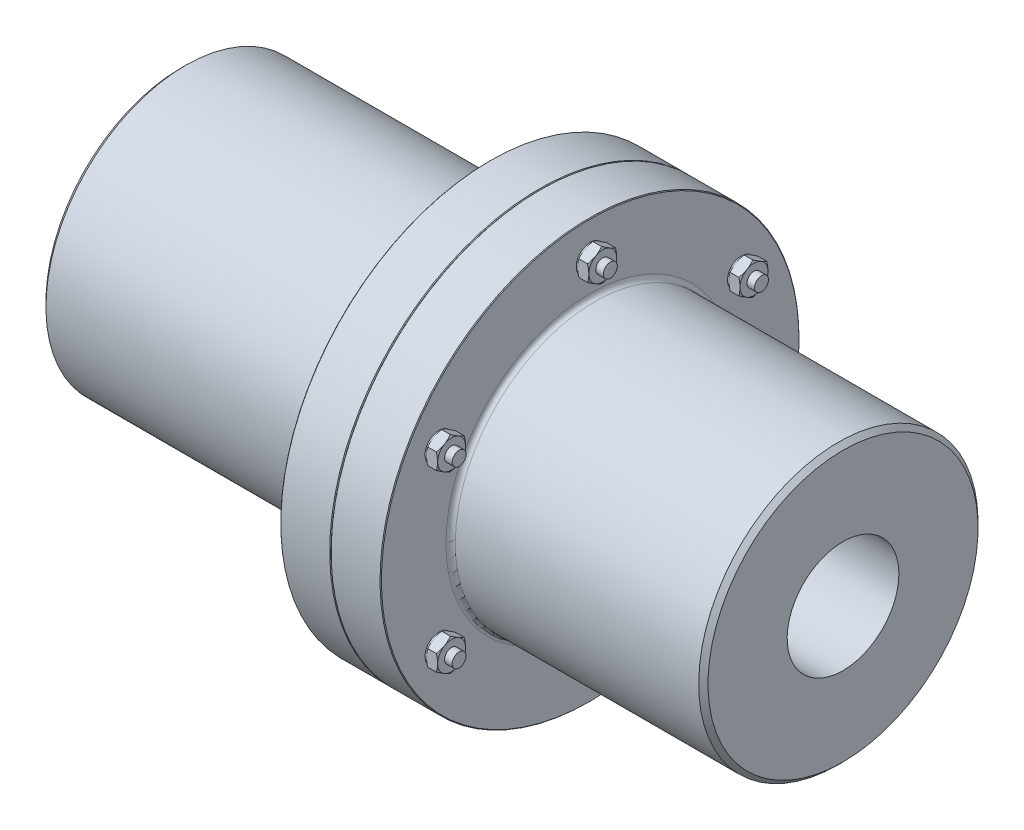
SolidWorks part; units mm, degrees
ref_plane "Front Plane" through (0, 0, 0) normal (0, 0, 1) x (1, 0, 0)
ref_plane "Top Plane" through (0, 0, 0) normal (0, 1, 0) x (1, 0, 0)
ref_plane "Right Plane" through (0, 0, 0) normal (1, 0, 0) x (0, 0, -1)
sketch "Sketch1" plane through (0, 0, 0) normal (0, 0, 1) x (1, 0, 0)
  line L0 (-257, 0) -> (217, 0) construction
  line L1 (0, 0) -> (0, 150) construction
  line L2 (36, 150) -> (-36, 150)
  line L3 (-36, 150) -> (-36, 100)
  line L4 (-36, 100) -> (-257, 100)
  line L5 (-257, 100) -> (-257, 0)
  line L6 (5, 105) -> (-5, 105)
  line L7 (-5, 105) -> (-5, 0)
  line L8 (-5, 65) -> (-257, 65)
  line L9 (-257, 66) -> (-256, 65)
  line L10 (-256, 65) -> (-256, 0)
  line L11 (-257, 2) -> (-5, 2)
  line L12 (36, 150) -> (36, 100)
  line L13 (217, 2) -> (5, 2)
  line L14 (216, 60) -> (216, 0)
  line L15 (217, 61) -> (216, 60)
  line L16 (5, 60) -> (217, 60)
  line L17 (5, 105) -> (5, 0)
  line L18 (217, 100) -> (217, 0)
  line L19 (36, 100) -> (217, 100)
  line L20 (-36, 125) -> (36, 125) construction
  line L21 (-36, 130) -> (36, 130)
  point P29 (0, 105)
  dimension "L" = 252
  dimension "S" = 10
  dimension "d1" = 130
  dimension "(D1)" = 200
  dimension "b" = 72
  dimension "D" = 300
  dimension "D22" = 250
  dimension "沉孔d1" = 210
  dimension "D4" = 1
  dimension "D5" = 45
  dimension "D6" = 4
  dimension "D7" = 1
  dimension "螺母d" = 10
  dimension "d2" = 120
  dimension "D8" = 45
  dimension "L2" = 212
sketch "Sketch14" plane through (0, 0, 0) normal (1, 0, 0) x (0, 0, -1)
  line L0 (0, 0) -> (-72.4, 0) construction
  line L1 (-72.4, 0) -> (-72.4, 16)
  line L2 (-72.4, 16) -> (-63, 16)
  line L3 (0, 0) -> (0, 150) construction
  line L4 (0, 0) -> (0, 150) construction
  line L6 (72.4, 16) -> (63, 16)
  line L7 (72.4, 0) -> (72.4, 16)
  line L8 (0, 0) -> (-36.2, -62.7002) construction
  line L9 (0, 0) -> (65, 0) construction
  line L10 (-36.2, -62.7002) -> (-50.0564, -54.7002)
  line L11 (-50.0564, -54.7002) -> (-45.3564, -46.5596)
  line L12 (0, 0) -> (32.5, 56.2917) construction
  circle A0 centre (0, 0) radius 65
  point P4 (-65, 0)
  point P12 (65, 0)
  dimension "D1" = 120
  dimension "b1" = 32
  dimension "t1" = 137.4
  dimension "B型t" = 137.4
  dimension "B型b" = 32
sketch "Sketch2" plane through (0, 0, 0) normal (0, 0, 1) x (1, 0, 0)
  line L0 (-257, 100) -> (-257, 0) construction
  line L1 (-36, 100) -> (-257, 100) construction
  line L2 (-36, 150) -> (-36, 100) construction
  line L3 (36, 150) -> (-36, 150) construction
  line L4 (0, 0) -> (0, 150) construction
  line L5 (5, 105) -> (-5, 105) construction
  line L6 (-5, 105) -> (-5, 0) construction
  line L8 (-257, 100) -> (-257, 0)
  line L9 (-36, 100) -> (-257, 100)
  line L10 (-36, 150) -> (-36, 100)
  line L11 (0, 150) -> (-36, 150)
  line L12 (0, 105) -> (0, 150)
  line L13 (0, 105) -> (-5, 105)
  line L14 (-5, 105) -> (-5, 0)
  line L15 (-257, 0) -> (-5, 0)
  line L18 (-257, 0) -> (217, 0) construction
  line L21 (-257, 0) -> (217, 0) construction
revolve "Revolve1" add sketch "Sketch2" angle 360 mid plane about L21
chamfer "Chamfer1" distance 3.3333 angle 45 1 edges at (-257, -100, 0)
chamfer "Chamfer2" distance 0.5 angle 45 2 edges at (0, -150, 0) (-36, -150, 0)
fillet "Fillet1" radius 1 1 edges at (-36, -100, 0)
sketch "Sketch15" plane through (0, 0, 0) normal (1, 0, 0) x (0, 0, -1)
  circle A0 centre (0, 0) radius 65 construction
  circle A1 centre (0, 0) radius 65
extrude "Cut-Extrude5" cut sketch "Sketch15" against normal through all
sketch "Sketch20" plane through (0, 0, 0) normal (1, 0, 0) x (0, 0, -1)
  line L0 (72.4, 16) -> (63, 16) construction
  line L1 (72.4, 0) -> (72.4, 16) construction
  line L2 (0, 0) -> (65, 0) construction
  line L3 (72.4, 16) -> (63, 16)
  line L4 (72.4, -16) -> (72.4, 16)
  line L5 (0, 0) -> (65, 0) construction
  line L6 (72.4, -16) -> (63, -16)
  circle A0 centre (0, 0) radius 65 construction
  circle A1 centre (0, 0) radius 65
extrude "Cut-Extrude7" cut sketch "Sketch20" against normal through all contours A1 L6 L4 L3
sketch "Sketch22" [suppressed] plane through (0, 0, 0) normal (1, 0, 0) x (0, 0, -1)
  line L0 (0, 0) -> (-6.15, -10.6521) construction
  line L1 (-8.7481, -9.1521) -> (-7.105, -6.3062) construction
  line L2 (-6.15, -10.6521) -> (-8.7481, -9.1521) construction
  line L3 (0, 0) -> (-6.15, -10.6521) construction
  line L4 (-8.7481, -9.1521) -> (-7.105, -6.3062)
  line L5 (-3.5519, -12.1521) -> (-8.7481, -9.1521)
  line L6 (-3.5519, -12.1521) -> (-1.9089, -9.3062)
  circle A0 centre (0, 0) radius 9.5 construction
  circle A1 centre (0, 0) radius 9.5
extrude "Cut-Extrude8" [suppressed] cut sketch "Sketch22" against normal through all contours L3 A1 L4 L5 | A1 L3 L5 L6
sketch "Sketch23" [suppressed] plane through (0, 0, 0) normal (1, 0, 0) x (0, 0, -1)
  line L0 (-12.3, 3) -> (-9.0139, 3) construction
  line L1 (-12.3, 0) -> (-12.3, 3) construction
  line L2 (0, 0) -> (-12.3, 0) construction
  line L3 (-12.3, 3) -> (-9.0139, 3)
  line L4 (-12.3, -3) -> (-12.3, 3)
  line L5 (0, 0) -> (-12.3, 0) construction
  line L6 (-12.3, -3) -> (-9.0139, -3)
  circle A0 centre (0, 0) radius 9.5 construction
  circle A1 centre (0, 0) radius 9.5
extrude "Cut-Extrude9" [suppressed] cut sketch "Sketch23" against normal through all contours L5 A1 L3 L4 | A1 L5 L4 L6
sketch "Sketch3" plane through (0, 0, 0) normal (0, 0, 1) x (1, 0, 0)
  line L0 (36, 150) -> (-36, 150) construction
  line L1 (36, 150) -> (36, 100) construction
  line L2 (36, 100) -> (217, 100) construction
  line L3 (217, 100) -> (217, 0) construction
  line L4 (5, 105) -> (-5, 105) construction
  line L5 (5, 105) -> (5, 0) construction
  line L9 (36, 150) -> (0, 150)
  line L10 (36, 150) -> (36, 100)
  line L11 (36, 100) -> (217, 100)
  line L12 (217, 100) -> (217, 60)
  line L13 (5, 105) -> (0, 105)
  line L14 (5, 105) -> (5, 0)
  line L15 (5, 0) -> (217, 0)
  line L16 (-257, 0) -> (217, 0) construction
  line L17 (217, 60) -> (217, 0)
  line L18 (0, 150) -> (0, 105)
  line L19 (-257, 0) -> (217, 0) construction
revolve "Revolve2" add sketch "Sketch3" angle 360 mid plane about L19
sketch "Sketch16" plane through (0, 0, 0) normal (1, 0, 0) x (0, 0, -1)
  line L0 (0, 0) -> (-33.7, -58.3701) construction
  line L1 (0, 0) -> (-150, 0) construction
  line L2 (-67.4, -16) -> (-67.4, 16) construction
  line L3 (-67.4, 16) -> (-57.8273, 16) construction
  line L4 (-67.4, -16) -> (-57.8273, -16) construction
  line L5 (0, 0) -> (0, 150) construction
  line L6 (0, 0) -> (0, 150) construction
  line L7 (67.4, -16) -> (57.8273, -16) construction
  line L8 (67.4, 16) -> (57.8273, 16) construction
  line L9 (67.4, -16) -> (67.4, 16) construction
  line L10 (0, 0) -> (67.4, 0) construction
  line L12 (-19.8436, -66.3701) -> (-47.5564, -50.3701) construction
  line L13 (-47.5564, -50.3701) -> (-42.7701, -42.0799) construction
  line L14 (-19.8436, -66.3701) -> (-15.0573, -58.0799) construction
  line L15 (0, 0) -> (30, 51.9615) construction
  circle A0 centre (0, 0) radius 60
  circle A1 centre (0, 0) radius 150 construction
  point P7 (-60, 0)
  point P12 (-67.4, 0)
  point P19 (67.4, 0)
  point P20 (60, 0)
  dimension "D1" = 120
  dimension "b2" = 32
  dimension "t2" = 127.4
  dimension "D2" = 32
  dimension "D3" = 127.4
extrude "Cut-Extrude6" cut sketch "Sketch16" along normal through all
sketch "Sketch24" plane through (0, 0, 0) normal (1, 0, 0) x (0, 0, -1)
  line L6 (67.4, 16) -> (57.8273, 16) construction
  line L7 (67.4, -16) -> (67.4, 16) construction
  line L8 (67.4, -16) -> (57.8273, -16) construction
  line L9 (67.4, 16) -> (57.8273, 16)
  line L10 (67.4, -16) -> (67.4, 16)
  line L11 (67.4, -16) -> (57.8273, -16)
  circle A0 centre (0, 0) radius 60 construction
  circle A1 centre (0, 0) radius 60
sketch "Sketch25" [suppressed] plane through (0, 0, 0) normal (1, 0, 0) x (0, 0, -1)
  line L0 (-8.7481, -9.1521) -> (-7.105, -6.3062) construction
  line L1 (-3.5519, -12.1521) -> (-8.7481, -9.1521) construction
  line L2 (-3.5519, -12.1521) -> (-1.9089, -9.3062) construction
  line L3 (-8.7481, -9.1521) -> (-7.105, -6.3062)
  line L4 (-3.5519, -12.1521) -> (-8.7481, -9.1521)
  line L5 (-3.5519, -12.1521) -> (-1.9089, -9.3062)
  circle A0 centre (0, 0) radius 9.5 construction
  circle A1 centre (0, 0) radius 9.5
extrude "Cut-Extrude11" [suppressed] cut sketch "Sketch25" along normal through all contours A1 L3 L4 L5
sketch "Sketch26" [suppressed] plane through (0, 0, 0) normal (1, 0, 0) x (0, 0, -1)
  line L6 (-12.3, 3) -> (-9.0139, 3) construction
  line L7 (-12.3, -3) -> (-12.3, 3) construction
  line L8 (-12.3, -3) -> (-9.0139, -3) construction
  line L9 (-12.3, 3) -> (-9.0139, 3)
  line L10 (-12.3, -3) -> (-12.3, 3)
  line L11 (-12.3, -3) -> (-9.0139, -3)
  circle A0 centre (0, 0) radius 9.5 construction
  circle A1 centre (0, 0) radius 9.5
extrude "Cut-Extrude12" [suppressed] cut sketch "Sketch26" along normal through all
chamfer "Chamfer3" distance 0.5 angle 45 2 edges at (36, -150, 0) (0, -150, 0)
chamfer "Chamfer4" distance 3.3333 angle 45 1 edges at (217, -100, 0)
fillet "Fillet2" radius 3.3333 1 edges at (36, -100, 0)
sketch "Sketch6" plane through (-36, 0, 0) normal (-1, 0, 0) x (0, 0, 1)
  circle A0 centre (0, 125) radius 5
extrude "Cut-Extrude1" cut sketch "Sketch6" against normal up to vertex (72 mm away) up to point (36, 150, 0)
chamfer "Chamfer5" distance 0.2 angle 45 1 edges at (-36, 125, 5)
chamfer "Chamfer6" distance 0.2 angle 45 1 edges at (36, 125, 5)
pattern_circular "CircPattern1" count 6 over 360 about axis through (0, 0, 0) along (1, 0, 0) of "Cut-Extrude1", "Chamfer5", "Chamfer6"
sketch "Sketch7" plane through (0, 0, 0) normal (0, 0, 1) x (1, 0, 0)
  line L0 (-36, 125) -> (-36, 130)
  line L1 (-36, 130) -> (50.4, 130)
  line L2 (50.4, 130) -> (50.4, 125)
  line L3 (50.4, 125) -> (-36, 125)
  line L4 (-36, 150) -> (-36, 100) construction
  dimension "D1" = 86.4
revolve "Revolve3" add sketch "Sketch7" angle 360 mid plane about L3
sketch "Sketch8" plane through (-36, 0, 0) normal (-1, 0, 0) x (0, 0, 1)
  line L1 (0, 136.547) -> (-10, 130.7735)
  line L2 (-10, 130.7735) -> (-10, 119.2265)
  line L3 (-10, 119.2265) -> (0, 113.453)
  line L4 (0, 113.453) -> (10, 119.2265)
  line L5 (10, 119.2265) -> (10, 130.7735)
  line L6 (10, 130.7735) -> (0, 136.547)
  circle A0 centre (0, 125) radius 10 construction
  dimension "D1" = 20
extrude "Boss-Extrude1" add sketch "Sketch8" along normal blind 8
sketch "Sketch9" plane through (-44, 0, 0) normal (-1, 0, 0) x (0, 0, 1)
  circle A0 centre (0, 125) radius 10 construction
  circle A1 centre (0, 125) radius 10
  circle A2 centre (0, 125) radius 15
  dimension "D1" = 30
extrude "Cut-Extrude2" cut sketch "Sketch9" against normal blind 1 draft 60
sketch "Sketch10" plane through (36, 0, 0) normal (1, 0, 0) x (0, 0, -1)
  circle A0 centre (0, 125) radius 10
  dimension "D1" = 20
extrude "Boss-Extrude2" add sketch "Sketch10" along normal blind 1
sketch "Sketch11" plane through (37, 0, 0) normal (1, 0, 0) x (0, 0, -1)
  line L6 (10, 130.7735) -> (0, 136.547)
  line L7 (10, 119.2265) -> (10, 130.7735)
  line L8 (0, 113.453) -> (10, 119.2265)
  line L9 (-10, 119.2265) -> (0, 113.453)
  line L10 (-10, 130.7735) -> (-10, 119.2265)
  line L11 (0, 136.547) -> (-10, 130.7735)
  line L12 (10, 130.7735) -> (0, 136.547)
  line L13 (10, 119.2265) -> (10, 130.7735)
  line L14 (0, 113.453) -> (10, 119.2265)
  line L15 (-10, 119.2265) -> (0, 113.453)
  line L16 (-10, 130.7735) -> (-10, 119.2265)
  line L17 (0, 136.547) -> (-10, 130.7735)
  dimension "D1" = 0
extrude "Boss-Extrude3" add sketch "Sketch11" along normal blind 8
sketch "Sketch12" plane through (45, 0, 0) normal (1, 0, 0) x (0, 0, -1)
  circle A1 centre (0, 125) radius 15
  circle A2 centre (0, 125) radius 15
  circle A3 centre (0, 125) radius 10
  circle A4 centre (0, 125) radius 10
  dimension "D1" = 0
  dimension "D2" = 0
extrude "Cut-Extrude3" cut sketch "Sketch12" against normal blind 1 draft 60
sketch "Sketch13" plane through (37, 0, 0) normal (-1, 0, 0) x (0, 0, 1)
  circle A1 centre (0, 125) radius 10
  circle A2 centre (0, 125) radius 10
  circle A3 centre (0, 125) radius 15
  circle A4 centre (0, 125) radius 15
  dimension "D1" = 0
  dimension "D2" = 0
extrude "Cut-Extrude4" cut sketch "Sketch13" against normal blind 1 draft 60
pattern_circular "CircPattern3" count 6 over 360 about axis through (0, 0, 0) along (1, 0, 0) of "Revolve3", "Boss-Extrude1", "Cut-Extrude2", "Boss-Extrude2", "Boss-Extrude3", "Cut-Extrude3", "Cut-Extrude4"
sketch "Sketch27" plane through (5, 0, 0) normal (-1, 0, 0) x (0, 0, 1)
  circle A0 centre (0, 0) radius 60
  circle A1 centre (0, 0) radius 40
  dimension "D1" = 80
extrude "Boss-Extrude4" add sketch "Sketch27" against normal blind 212
